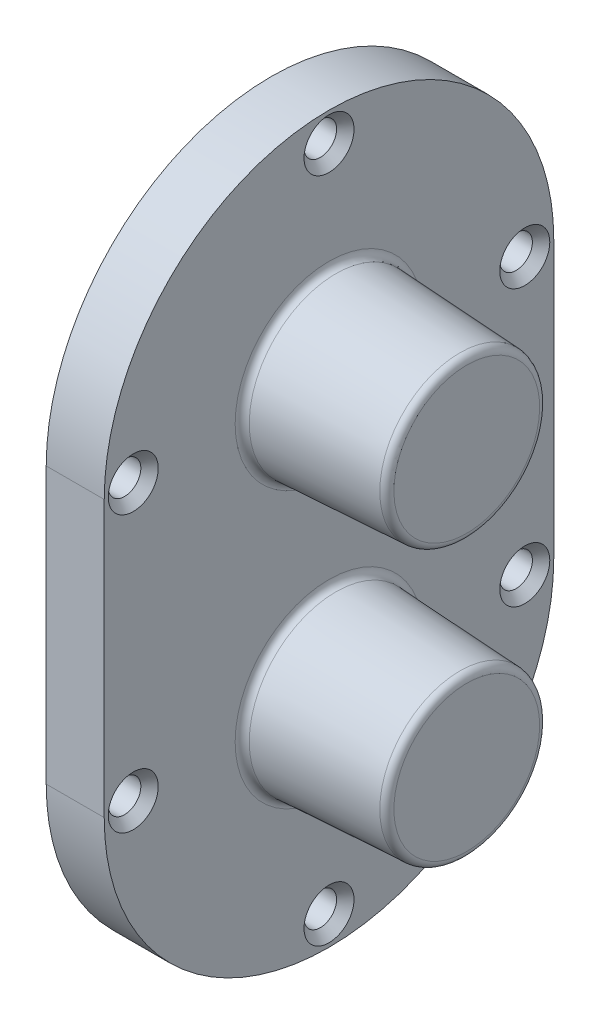
from build123d import *

# Parameters (mm, degrees)
BOSS_EXTRUDE1_DEPTH            = 8
F_16_0_16_DIAMETER_HOLE1_D     = 16
F_16_0_16_DIAMETER_HOLE1_DEPTH = 24
F_4_5_4_5_DIAMETER_HOLE1_D     = 4.5
CHAMFER1_SIZE                  = 1.2
FILLET1_R                      = 1


with BuildPart() as part:
    # Sketch1 → Boss-Extrude1 (new body)
    with BuildSketch(Plane(origin=(8, 0, 0), x_dir=(0, 0, -1), z_dir=(1, 0, 0))):
        with BuildLine():
            Line((31, -19), (31, 19))
            ThreePointArc((31, 19), (0, 50), (-31, 19))
            Line((-31, 19), (-31, -19))
            ThreePointArc((-31, -19), (0, -50), (31, -19))
        make_face()
    extrude(amount=-BOSS_EXTRUDE1_DEPTH)

    # Sketch2 → Revolve1 (revolve)
    with BuildSketch(Plane.XY, mode=Mode.PRIVATE) as revolve1_sk:
        Polygon((8, -7.004252194), (8, -19), (27, -19), (27, -8), align=None)
    revolve(revolve1_sk.sketch.rotate(Axis((8, -19, 0), (1, 0, 0)), 270), axis=Axis((8, -19, 0), (1, 0, 0)))

    # Sketch3 → Revolve2 (revolve)
    with BuildSketch(Plane.XY, mode=Mode.PRIVATE) as revolve2_sk:
        Polygon((8, 30.995747806), (8, 19), (27, 19), (27, 30), align=None)
    revolve(revolve2_sk.sketch.rotate(Axis((8, 19, 0), (1, 0, 0)), 270), axis=Axis((8, 19, 0), (1, 0, 0)))

    # Ø16.0 (16) Diameter Hole1
    with Locations(Plane.ZY):
        with Locations((0, 19), (0, -19)):
            Hole(F_16_0_16_DIAMETER_HOLE1_D / 2, depth=F_16_0_16_DIAMETER_HOLE1_DEPTH)

    # Ø4.5 (4.5) Diameter Hole1 (through all)
    with Locations(Plane(origin=(8, 0, 0), x_dir=(0, 0, -1), z_dir=(1, 0, 0))):
        with Locations((0, 46), (-27, 19), (27, 19), (-27, -19), (27, -19), (0, -46)):
            Hole(F_4_5_4_5_DIAMETER_HOLE1_D / 2)

    # Chamfer1
    chamfer1_edges = [part.edges().sort_by_distance(p)[0] for p in [
        (8, -46, -2.25),
        (8, -19, -29.25),
        (8, -19, 24.75),
        (8, 19, -29.25),
        (8, 19, 24.75),
        (8, 46, -2.25),
    ]]
    chamfer(chamfer1_edges, length=CHAMFER1_SIZE)

    # Fillet1
    fillet1_edges = [part.edges().sort_by_distance(p)[0] for p in [
        (8, -19, 11.995747806),
        (27, -19, 11),
        (8, 19, 11.995747806),
        (27, 19, 11),
    ]]
    fillet(fillet1_edges, radius=FILLET1_R)


solid = part.part
